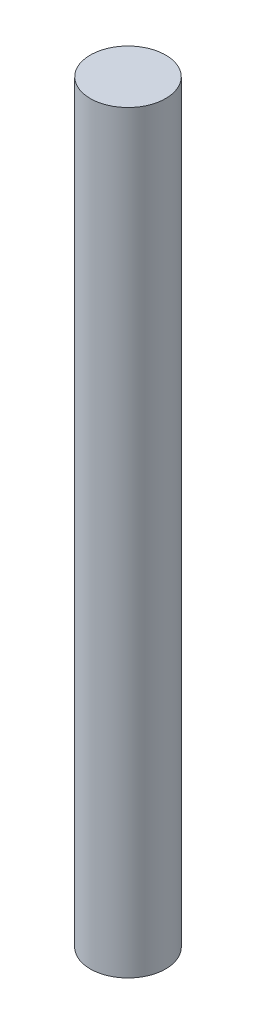
from build123d import *

# Parameters (mm, degrees)
SKETCH1_R             = 10
BOSS_EXTRUDE1_DEPTH   = 200
M6_TAPPED_HOLE1_D     = 5
M6_TAPPED_HOLE1_DEPTH = 15
M6_TAPPED_HOLE1_TIP   = 1.502151548


with BuildPart() as part:
    # Sketch1 → Boss-Extrude1 (new body)
    with BuildSketch(Plane(origin=(0, 0, 0), x_dir=(1, 0, 0), z_dir=(0, 1, 0))):
        with Locations(Location((0, 0, 0), (0, 0, 270))):
            Circle(SKETCH1_R)
    extrude(amount=BOSS_EXTRUDE1_DEPTH)

    # M6 Tapped Hole1
    with Locations(Plane(origin=(0, 0, 0), x_dir=(-1, 0, 0), z_dir=(0, -1, 0))):
        with Locations((0, 0)):
            Hole(M6_TAPPED_HOLE1_D / 2, depth=M6_TAPPED_HOLE1_DEPTH)
            with Locations((0, 0, -(M6_TAPPED_HOLE1_DEPTH + M6_TAPPED_HOLE1_TIP / 2))):  # 118° drill point
                Cone(0, M6_TAPPED_HOLE1_D / 2, M6_TAPPED_HOLE1_TIP, mode=Mode.SUBTRACT)


solid = part.part
